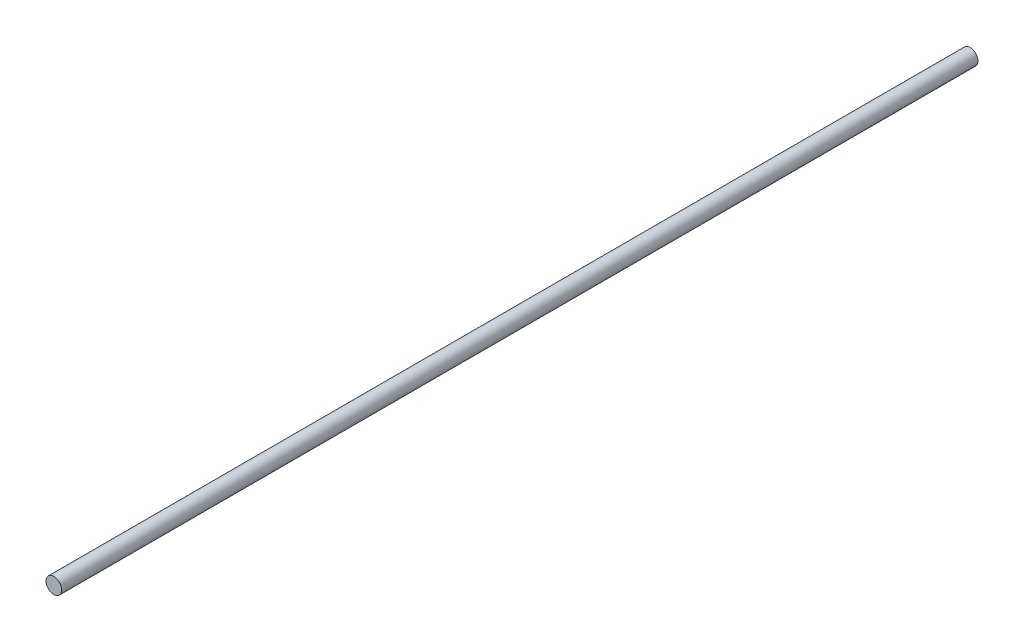
SolidWorks part; units mm, degrees
ref_plane "Front Plane" through (0, 0, 0) normal (0, 0, 1) x (1, 0, 0)
ref_plane "Top Plane" through (0, 0, 0) normal (0, 1, 0) x (1, 0, 0)
ref_plane "Right Plane" through (0, 0, 0) normal (1, 0, 0) x (0, 0, -1)
sketch "Sketch1" plane through (0, 0, 0) normal (0, 0, 1) x (1, 0, 0)
  circle A0 centre (0, 0) radius 3
extrude "Boss-Extrude1" add sketch "Sketch1" along normal blind 350
